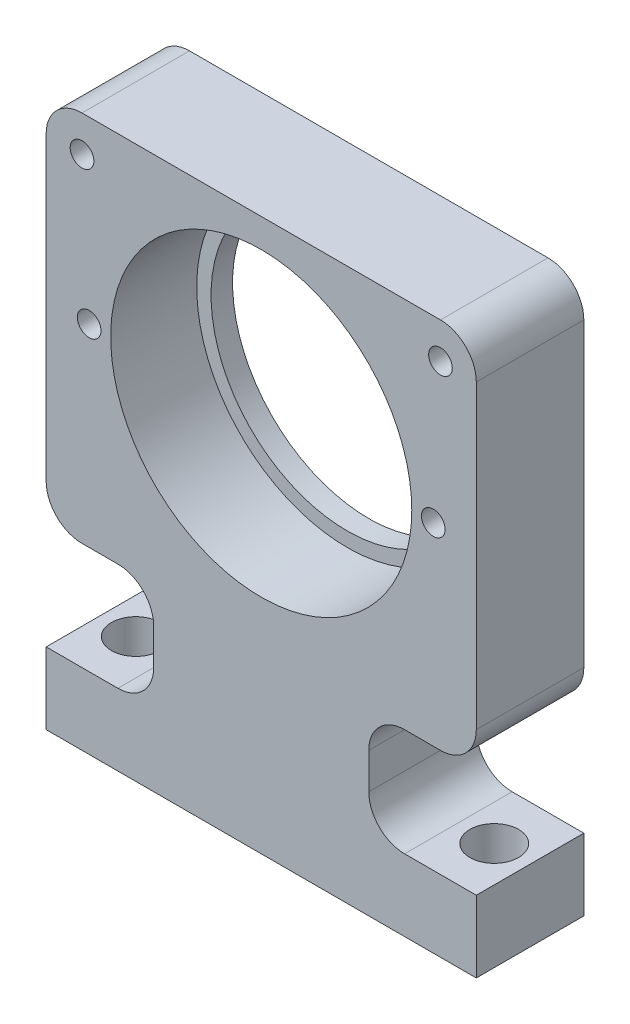
SolidWorks part; units mm, degrees
material "6061合金"
ref_plane "Front Plane" through (0, 0, 0) normal (0, 0, 1) x (1, 0, 0)
ref_plane "Top Plane" through (0, 0, 0) normal (0, 1, 0) x (1, 0, 0)
ref_plane "Right Plane" through (0, 0, 0) normal (1, 0, 0) x (0, 0, -1)
sketch "Sketch1" plane through (0, 0, 0) normal (0, 0, 1) x (1, 0, 0)
  line L0 (0, 0) -> (0, 77) construction
  line L1 (30, 0) -> (-30, 0)
  line L2 (-30, 0) -> (-30, 10)
  line L3 (-30, 10) -> (-15, 10)
  line L4 (-15, 10) -> (-15, 25)
  line L5 (-15, 25) -> (-30, 25)
  line L6 (-30, 25) -> (-30, 77)
  line L7 (-30, 77) -> (30, 77)
  line L8 (30, 25) -> (30, 77)
  line L9 (15, 25) -> (30, 25)
  line L10 (15, 10) -> (15, 25)
  line L11 (30, 10) -> (15, 10)
  line L12 (30, 0) -> (30, 10)
  dimension "D1" = 77
  dimension "D2" = 60
  dimension "D3" = 10
  dimension "D4" = 15
  dimension "D5" = 15
extrude "Boss-Extrude1" add sketch "Sketch1" along normal mid plane 15
sketch "Sketch2" plane through (0, 0, 0) normal (0, -1, 0) x (1, 0, 0)
  line L0 (-30, 0) -> (0, 0) construction
  line L1 (-30, 7.5) -> (-30, -7.5) construction
  line L2 (0, 0) -> (0, 13.2182) construction
  circle A0 centre (-25, 0) radius 3.4
  circle A1 centre (25, 0) radius 3.4
  dimension "D1" = 5
  dimension "D2" = 6.8
extrude "Cut-Extrude1" cut sketch "Sketch2" against normal blind 15
sketch "Sketch3" plane through (0, 0, 7.5) normal (0, 0, 1) x (1, 0, 0)
  line L0 (0, 0) -> (0, 52) construction
  line L1 (-30, 0) -> (30, 0) construction
  circle A0 centre (0, 52) radius 21
  dimension "D1" = 42
  dimension "D2" = 52
sketch "Sketch4" plane through (0, 0, 7.5) normal (0, 0, 1) x (1, 0, 0)
  line L0 (-30, 0) -> (30, 0) construction
  line L1 (0, 0) -> (0, 52) construction
  circle A0 centre (0, 52) radius 19
  dimension "D1" = 38
  dimension "D2" = 52
extrude "Cut-Extrude3" cut sketch "Sketch4" against normal through all
extrude "Cut-Extrude4" cut sketch "Sketch3" against normal blind 12
hole_wizard "M4 Tapped Hole2" positions "Sketch7" profile "Sketch8" tap size "M4" standard "GB" end condition through all
sketch "Sketch7" plane through (0, 0, 7.5) normal (0, 0, 1) x (1, 0, 0)
  line L0 (24, 52) -> (0, 52) construction
  line L2 (-24, 52) -> (0, 52) construction
  point P0 (24, 52)
  point P2 (-24, 52)
  dimension "D1" = 24
  dimension "D2" = 24
cosmetic thread "Hole Thread1" parameters "D2"=4
cosmetic thread "Hole Thread2" parameters "D2"=4
sketch "Sketch8" plane through (24, 52, 7.5) normal (1, 0, 0) x (0, -1, 0)
  line L0 (0, 0) -> (0, 15)
  line L1 (0, 15) -> (1.65, 15)
  line L2 (1.65, 15) -> (1.65, 0)
  line L5 (1.65, 0) -> (0, 0)
  line L11 (0, -6.35) -> (0, 107.95) construction
  dimension "通孔螺纹孔钻头直径" = 3.3
  dimension "通孔螺纹孔钻头深度" = 15
hole_wizard "M4 Tapped Hole1" positions "Sketch9" profile "Sketch10" tap size "M4" standard "GB" end condition through all
sketch "Sketch9" plane through (0, 0, 7.5) normal (0, 0, 1) x (1, 0, 0)
  line L0 (0, 0) -> (0, 77) construction
  line L2 (30, 77) -> (-30, 77) construction
  line L3 (0, 52) -> (-11.0606, 52) construction
  point P0 (-25, 72)
  point P2 (25, 72)
  dimension "D1" = 25
  dimension "D2" = 20
cosmetic thread "Hole Thread3" parameters "D2"=4
cosmetic thread "Hole Thread4" parameters "D2"=4
sketch "Sketch10" plane through (-25, 72, 7.5) normal (1, 0, 0) x (0, -1, 0)
  line L0 (0, 0) -> (0, 15)
  line L1 (0, 15) -> (1.65, 15)
  line L2 (1.65, 15) -> (1.65, 0)
  line L5 (1.65, 0) -> (0, 0)
  line L11 (0, -6.35) -> (0, 107.95) construction
  dimension "通孔螺纹孔钻头直径" = 3.3
  dimension "通孔螺纹孔钻头深度" = 15
fillet "Fillet2" radius 5 8 edges at (-30, 25, 0) (30, 77, 0) (30, 25, 0) (15, 25, 0) (15, 10, 0) (-15, 10, 0) (-15, 25, 0) (-30, 77, 0)
